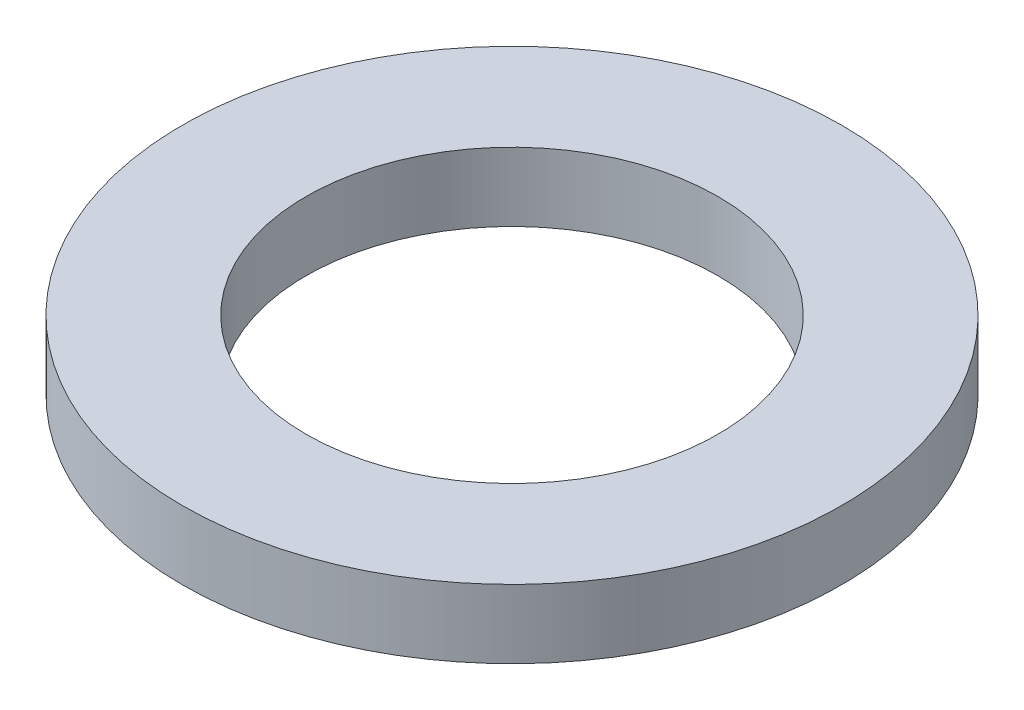
from build123d import *

# Parameters (mm, degrees)
SKETCH1_W = 4.5
SKETCH1_H = 2.5


with BuildPart() as part:
    # Sketch1 → Boss-Revolve (revolve)
    with BuildSketch(Plane.XY, mode=Mode.PRIVATE) as boss_revolve_sk:
        with Locations((-9.75, 9.894507042)):
            Rectangle(SKETCH1_W, SKETCH1_H)
    revolve(boss_revolve_sk.sketch.rotate(Axis((0, 0, 0), (0, 1, 0)), 270), axis=Axis((0, 0, 0), (0, 1, 0)))


solid = part.part
